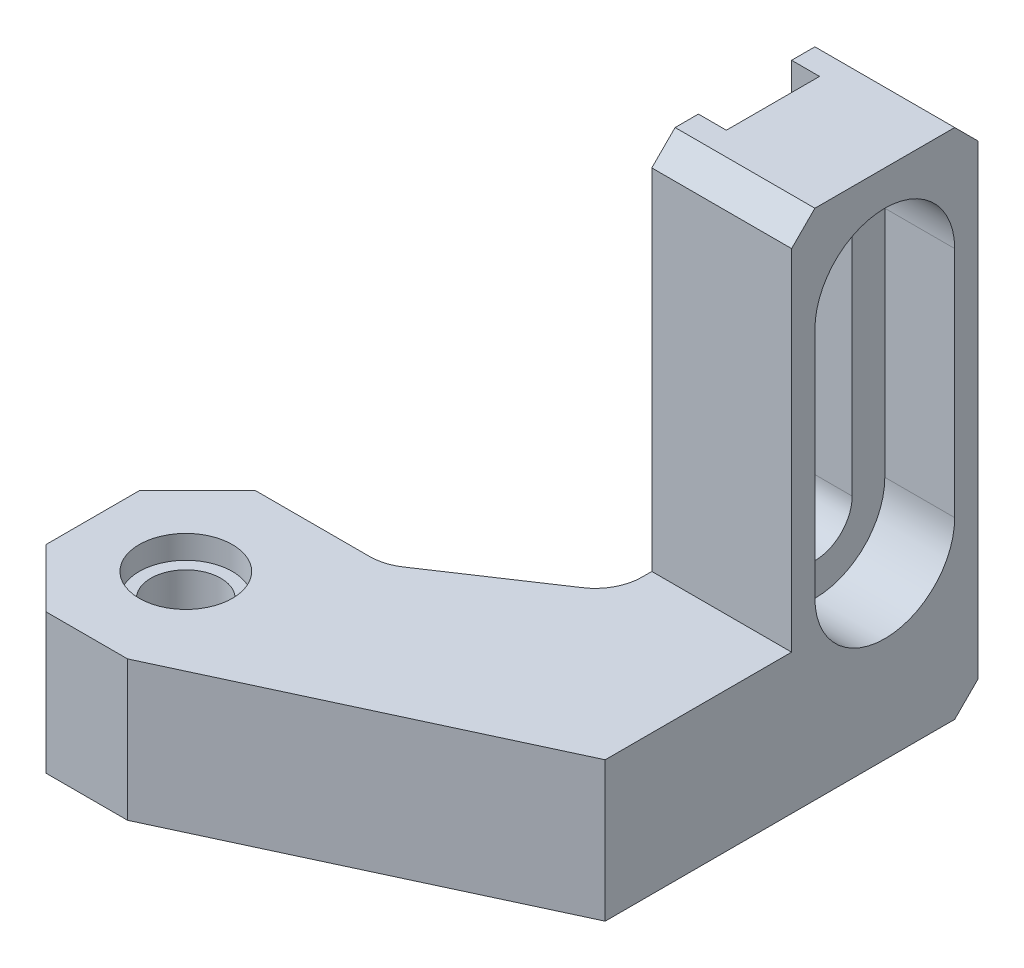
SolidWorks part; units mm, degrees
ref_plane "Front Plane" through (0, 0, 0) normal (0, 0, 1) x (1, 0, 0)
ref_plane "Top Plane" through (0, 0, 0) normal (0, 1, 0) x (1, 0, 0)
ref_plane "Right Plane" through (0, 0, 0) normal (1, 0, 0) x (0, 0, -1)
sketch "Sketch1" plane through (0, 0, 0) normal (0, 0, 1) x (1, 0, 0)
  line L1 (-10, -11) -> (10, -11)
  line L2 (-10, -11) -> (-10, 11)
  line L3 (-10, 11) -> (10, 11)
  line L4 (10, -11) -> (10, 11)
  line L5 (-10, -11) -> (10, 11) construction
  line L6 (-10, 11) -> (10, -11) construction
  point P0 (0, 0)
  dimension "D1" = 20
  dimension "D2" = 22
extrude "Boss-Extrude1" add sketch "Sketch1" along normal blind 8
sketch "Sketch2" plane through (0, 0, 8) normal (0, 0, 1) x (1, 0, 0)
  line L0 (10, -11) -> (10, 11) construction
  line L1 (-10, -11) -> (10, -11)
  line L2 (-10, -11) -> (-10, -5)
  line L3 (-10, -5) -> (10, -5)
  line L4 (10, -11) -> (10, -5)
  dimension "D1" = 6
extrude "Boss-Extrude2" add sketch "Sketch2" along normal blind 14.5
sketch "Sketch4" plane through (0, -11, 0) normal (0, 1, 0) x (1, 0, 0)
  line L0 (-10, -22.5) -> (-10, -8) construction
  line L1 (10, -8) -> (-10, -8) construction
  circle A0 centre (-6, -18) radius 3.25
  dimension "D1" = 6.5
  dimension "D2" = 10
  dimension "D3" = 4
extrude "Cut-Extrude2" cut sketch "Sketch4" along normal offset from surface (5 mm away) 1 up to face at (2.5, -5, 18.875)
sketch "Sketch5" plane through (0, -11, 0) normal (0, 1, 0) x (1, 0, 0)
  circle A0 centre (-6, -18) radius 3.25
  circle A1 centre (-6, -18) radius 1.5
  circle A2 centre (-6, -18) radius 3.25 construction
  dimension "D1" = 3
extrude "Boss-Extrude3" add sketch "Sketch5" along normal up to surface (5 mm away) separate body up to face at (-6, -6, 14.75)
sketch "Sketch6" plane through (0, -11, 0) normal (0, -1, 0) x (1, 0, 0)
  line L1 (4, 0) -> (-10, 0)
  line L2 (4, 0) -> (4, 13.5)
  line L3 (4, 13.5) -> (-10, 13.5)
  line L4 (-10, 0) -> (-10, 13.5)
  line L6 (-10, 22.5) -> (-10, 0) construction
  line L7 (-10, 0) -> (10, 0) construction
  line L8 (10, 22.5) -> (10, 0) construction
  dimension "D1" = 6
  dimension "D2" = 13.5
extrude "Cut-Extrude3" cut sketch "Sketch6" against normal through all
sketch "Sketch7" plane through (4, 0, 0) normal (-1, 0, 0) x (0, 0, 1)
  line L0 (0, -11) -> (13.5, -11) construction
  line L1 (6, -11) -> (2, -11)
  line L2 (6, -11) -> (6, 11)
  line L3 (6, 11) -> (2, 11)
  line L4 (2, -11) -> (2, 11)
  line L5 (0, 11) -> (8, 11) construction
  line L6 (0, 11) -> (0, -11) construction
  dimension "D1" = 4
  dimension "D2" = 2
extrude "Cut-Extrude4" cut sketch "Sketch7" against normal blind 1.2
sketch "Sketch8" plane through (0, -11, 0) normal (0, -1, 0) x (1, 0, 0)
  line L0 (-4, 22.5) -> (10, 16)
  line L1 (-10, 22.5) -> (10, 22.5) construction
  line L2 (10, 22.5) -> (10, 0) construction
  line L3 (10, 16) -> (10, 22.5)
  line L4 (10, 22.5) -> (-4, 22.5)
  line L5 (4, 0) -> (10, 0) construction
  line L6 (-10, 22.5) -> (-10, 13.5) construction
  dimension "D1" = 16
  dimension "D2" = 6
extrude "Cut-Extrude5" cut sketch "Sketch8" against normal through all
sketch "Sketch11" plane through (10, 0, 0) normal (1, 0, 0) x (0, 0, -1)
  line L0 (-4, -3.5) -> (-4, 6.5) construction
  line L1 (-5.6, -3.5) -> (-5.6, 6.5)
  line L2 (-2.4, -3.5) -> (-2.4, 6.5)
  line L3 (-8, 11) -> (0, 11) construction
  line L4 (0, -11) -> (0, 11) construction
  arc A0 (-5.6, -3.5) -> (-2.4, -3.5) centre (-4, -3.5) ccw
  arc A1 (-2.4, 6.5) -> (-5.6, 6.5) centre (-4, 6.5) ccw
  point P2 (-4, 1.5)
  dimension "D1" = 3.2
  dimension "D2" = 10
  dimension "D3" = 4.5
  dimension "D4" = 4
extrude "Cut-Extrude6" cut sketch "Sketch11" against normal through all
sketch "Sketch12" plane through (10, 0, 0) normal (1, 0, 0) x (0, 0, -1)
  line L0 (-4, -3.5) -> (-4, 6.5) construction
  line L1 (-7, -3.5) -> (-7, 6.5)
  line L2 (-1, -3.5) -> (-1, 6.5)
  arc A0 (-7, -3.5) -> (-1, -3.5) centre (-4, -3.5) ccw
  arc A1 (-1, 6.5) -> (-7, 6.5) centre (-4, 6.5) ccw
  point P4 (-4, 1.5)
  dimension "D1" = 6
extrude "Cut-Extrude7" cut sketch "Sketch12" against normal blind 3
chamfer "Chamfer3" distance 2.5 angle 45 2 edges at (-10, -8, 22.5) (-10, -8, 13.5)
chamfer "Chamfer4" distance 1 angle 45 3 edges at (7, 11, 8) (7, 11, 0) (7, -11, 0)
sketch "Sketch13" plane through (0, -11, 0) normal (0, -1, 0) x (1, 0, 0)
  line L0 (-2, 13.5) -> (4, 9.5)
  line L1 (4, 13.5) -> (-7.5, 13.5) construction
  line L2 (4, 1) -> (4, 2) construction
  line L3 (4, 9.5) -> (4, 13.5)
  line L4 (4, 13.5) -> (-2, 13.5)
  line L5 (-10, 20) -> (-10, 16) construction
  dimension "D1" = 8
  dimension "D2" = 4
extrude "Boss-Extrude4" add sketch "Sketch13" against normal up to surface (6 mm away) up to face at (-0.8889, -5, 16.2222)
fillet "Fillet2" radius 2 2 edges at (-2, -8, 13.5) (4, -8, 9.5)
sketch "Sketch14" plane through (0, -11, 0) normal (0, -1, 0) x (1, 0, 0)
  circle A0 centre (-6, 18) radius 1.5
  circle A1 centre (-6, 18) radius 1.5 construction
extrude "Cut-Extrude8" cut sketch "Sketch14" against normal through all
sketch "Sketch15" plane through (0, -5, 0) normal (0, 1, 0) x (1, 0, 0)
  circle A0 centre (-6, -18) radius 2
  dimension "D1" = 4
extrude "Cut-Extrude9" cut sketch "Sketch15" against normal blind 1
